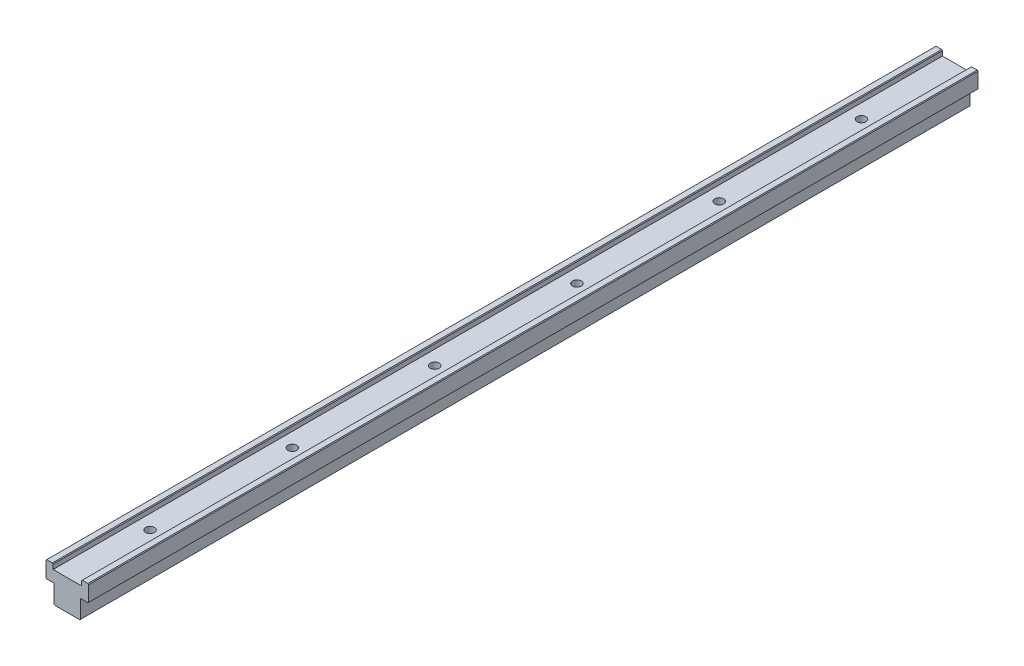
from build123d import *

# Parameters (mm, degrees)
BOSS_EXTRUDE1_DEPTH = 125
M3_TAPPED_HOLE1_D   = 2.5
CHAMFER1_SIZE       = 0.2
LPATTERN1_COUNT     = 6
LPATTERN1_PITCH     = 40


with BuildPart() as part:
    # Sketch1 → Boss-Extrude1 (new, symmetric)
    with BuildSketch(Plane.XY):
        Polygon((4, 0), (-4, 0), (-4, 1.5), (-6, 1.5), (-6, -3.2), (-3.7, -3.2), (-3.7, -8.5), (3.7, -8.5), (3.7, -3.2), (6, -3.2), (6, 1.5), (4, 1.5), align=None)
    extrude(amount=BOSS_EXTRUDE1_DEPTH, both=True)

    # M3 Tapped Hole1 (through all)
    with Locations(Plane(origin=(0, 0, 0), x_dir=(1, 0, 0), z_dir=(0, 1, 0))):
        with Locations((0, 98.25)):
            m3_tapped_hole1 = Hole(M3_TAPPED_HOLE1_D / 2)

    # Chamfer1
    chamfer1_edges = [part.edges().sort_by_distance(p)[0] for p in [
        (4, 1.5, 0),
        (6, 1.5, 0),
        (6, -3.2, 0),
        (3.7, -8.5, 0),
        (-3.7, -8.5, 0),
        (-6, -3.2, 0),
        (-6, 1.5, 0),
        (-4, 1.5, 0),
    ]]
    chamfer(chamfer1_edges, length=CHAMFER1_SIZE)

    # LPattern1: M3 Tapped Hole1 ×6
    with Locations(*[(0, 0, i * LPATTERN1_PITCH) for i in range(1, LPATTERN1_COUNT)]):
        add(m3_tapped_hole1, mode=Mode.SUBTRACT)


solid = part.part
